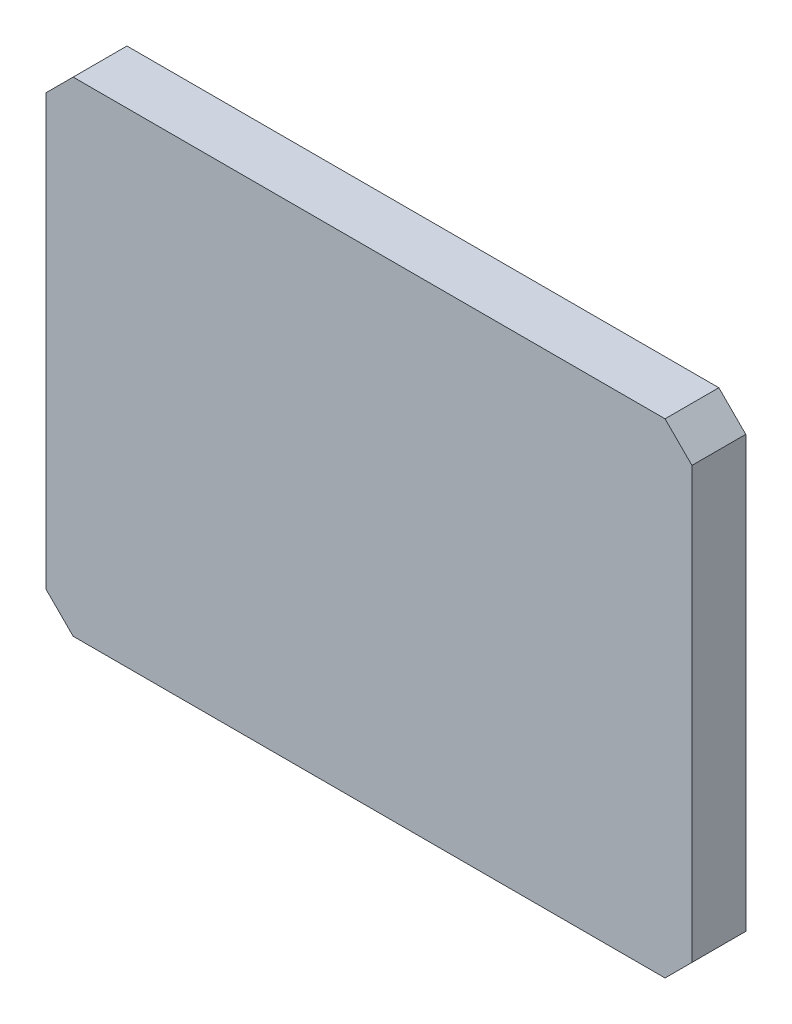
SolidWorks part; units mm, degrees
material "1023 Carbon Steel Plate (SS)"
ref_plane "Front Plane" through (0, 0, 0) normal (0, 0, 1) x (1, 0, 0)
ref_plane "Top Plane" through (0, 0, 0) normal (0, 1, 0) x (1, 0, 0)
ref_plane "Right Plane" through (0, 0, 0) normal (1, 0, 0) x (0, 0, -1)
sketch "Sketch1" plane through (0, 0, 0) normal (0, 0, 1) x (1, 0, 0)
  line L1 (60, 45) -> (-60, 45)
  line L2 (60, 45) -> (60, -45)
  line L3 (60, -45) -> (-60, -45)
  line L4 (-60, 45) -> (-60, -45)
  line L5 (60, 45) -> (-60, -45) construction
  line L6 (60, -45) -> (-60, 45) construction
  point P0 (0, 0)
  dimension "D1" = 120
  dimension "D2" = 90
extrude "Boss-Extrude1" add sketch "Sketch1" along normal blind 10
chamfer "Chamfer1" distance 5 angle 45 4 edges at (60, -45, 5) (-60, -45, 5) (-60, 45, 5) (60, 45, 5)
